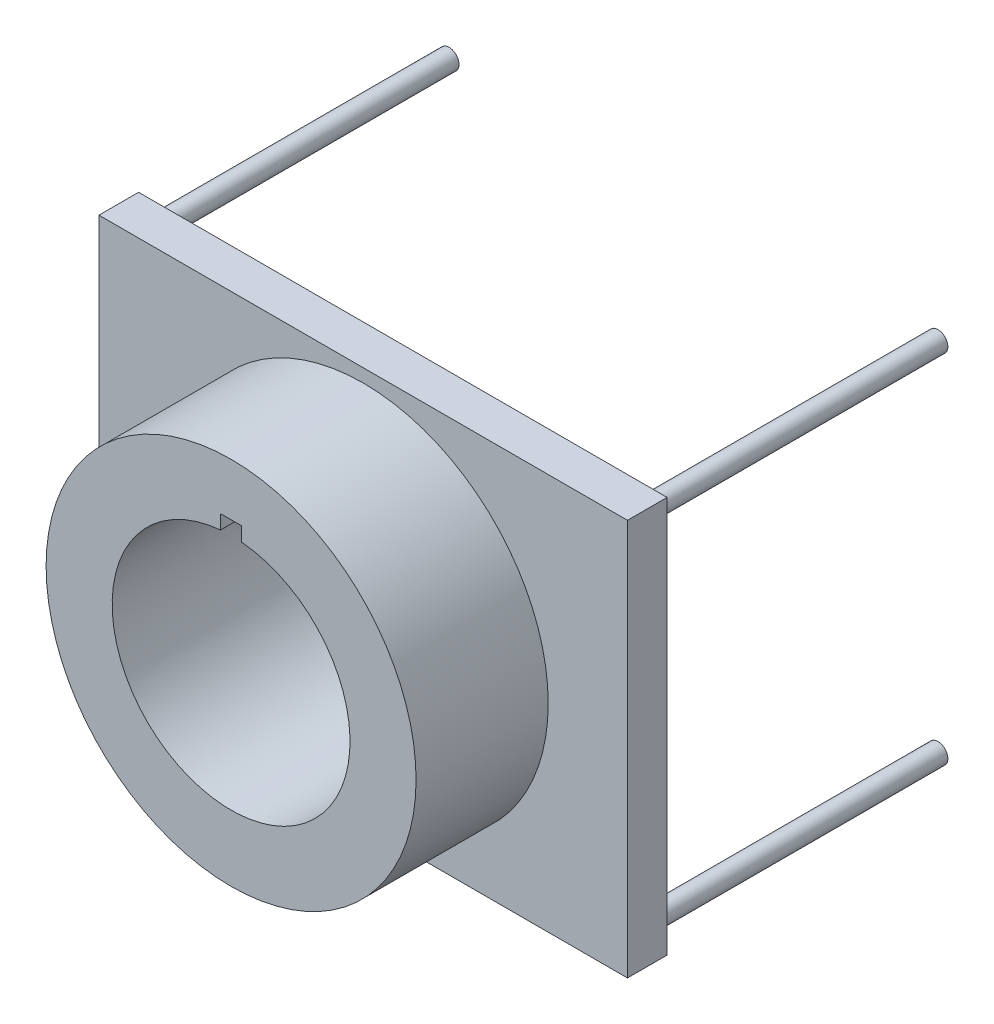
SolidWorks part; units mm, degrees
material "普通碳钢"
ref_plane "Front Plane" through (0, 0, 0) normal (0, 0, 1) x (1, 0, 0)
ref_plane "Top Plane" through (0, 0, 0) normal (0, 1, 0) x (1, 0, 0)
ref_plane "Right Plane" through (0, 0, 0) normal (1, 0, 0) x (0, 0, -1)
sketch "Sketch2" plane through (0, 0, 0) normal (0, 0, 1) x (1, 0, 0)
  circle A0 centre (0, 0) radius 45
  circle A1 centre (0, 0) radius 70
extrude "Boss-Extrude1" add sketch "Sketch2" along normal blind 50
sketch "Sketch3" plane through (0, 0, 0) normal (0, 0, -1) x (-1, 0, 0)
  line L1 (-100, -75) -> (100, -75)
  line L2 (-100, -75) -> (-100, 75)
  line L3 (-100, 75) -> (100, 75)
  line L4 (100, -75) -> (100, 75)
  line L5 (-100, -75) -> (100, 75) construction
  line L6 (-100, 75) -> (100, -75) construction
  point P0 (0, 0)
  dimension "D1" = 200
  dimension "D2" = 150
extrude "Boss-Extrude2" add sketch "Sketch3" along normal blind 15
sketch "Sketch4" plane through (0, 0, -15) normal (0, 0, -1) x (-1, 0, 0)
  line L0 (100, 75) -> (-100, 75) construction
  line L1 (-100, 75) -> (-100, -75) construction
  line L2 (0, 75) -> (0, -75) construction
  line L3 (-100, -75) -> (100, -75) construction
  line L4 (-100, 0) -> (100, 0) construction
  line L5 (100, -75) -> (100, 75) construction
  circle A0 centre (-92.5, 67.5) radius 3.75
  circle A1 centre (92.5, 67.5) radius 3.75
  circle A2 centre (92.5, -67.5) radius 3.75
  circle A3 centre (-92.5, -67.5) radius 3.75
  dimension "D3" = 7.5
  dimension "D1" = 7.5
  dimension "D2" = 7.5
extrude "Boss-Extrude3" add sketch "Sketch4" along normal blind 110
sketch "Sketch5" plane through (0, 0, 50) normal (0, 0, 1) x (1, 0, 0)
  line L0 (0, 75) -> (0, -75) construction
  line L1 (-100, 75) -> (100, 75) construction
  line L2 (100, -75) -> (-100, -75) construction
  line L4 (-4, 50.18) -> (4, 50.18)
  line L5 (-4, 50.18) -> (-4, 43.18)
  line L6 (4, 50.18) -> (4, 43.18)
  line L7 (-4, 43.18) -> (4, 43.18)
  circle A4 centre (0, 0) radius 45 construction
  point P13 (0, 50.18)
  dimension "D1" = 5.18
  dimension "D2" = 8
  dimension "D3" = 7
extrude "Cut-Extrude1" cut sketch "Sketch5" against normal up to surface (50 mm away) up to face at (70, 0, 0)
sketch "Sketch6" plane through (0, 0, 0) normal (0, 0, 1) x (1, 0, 0)
  circle A0 centre (0, 0) radius 70
  circle M2 centre (0, 0) radius 70
extrude "Cut-Extrude3" cut sketch "Sketch6" against normal blind 70 contours M2
sketch "Sketch9" plane through (0, 0, 0) normal (0, 0, -1) x (-1, 0, 0)
  line L0 (4, 44.8219) -> (4, 50.18) construction
  line L1 (4, 50.18) -> (-4, 50.18) construction
  line L2 (-4, 50.18) -> (-4, 44.8219) construction
  line L3 (4, 44.8219) -> (4, 50.18)
  line L4 (4, 50.18) -> (-4, 50.18)
  line L5 (-4, 50.18) -> (-4, 44.8219)
  arc A0 (-4, 44.8219) -> (4, 44.8219) centre (0, 0) ccw construction
  circle A1 centre (0, 0) radius 70 construction
  arc A2 (-4, 44.8219) -> (4, 44.8219) centre (0, 0) ccw
  circle A3 centre (0, 0) radius 70
extrude "Boss-Extrude4" add sketch "Sketch9" along normal blind 15
